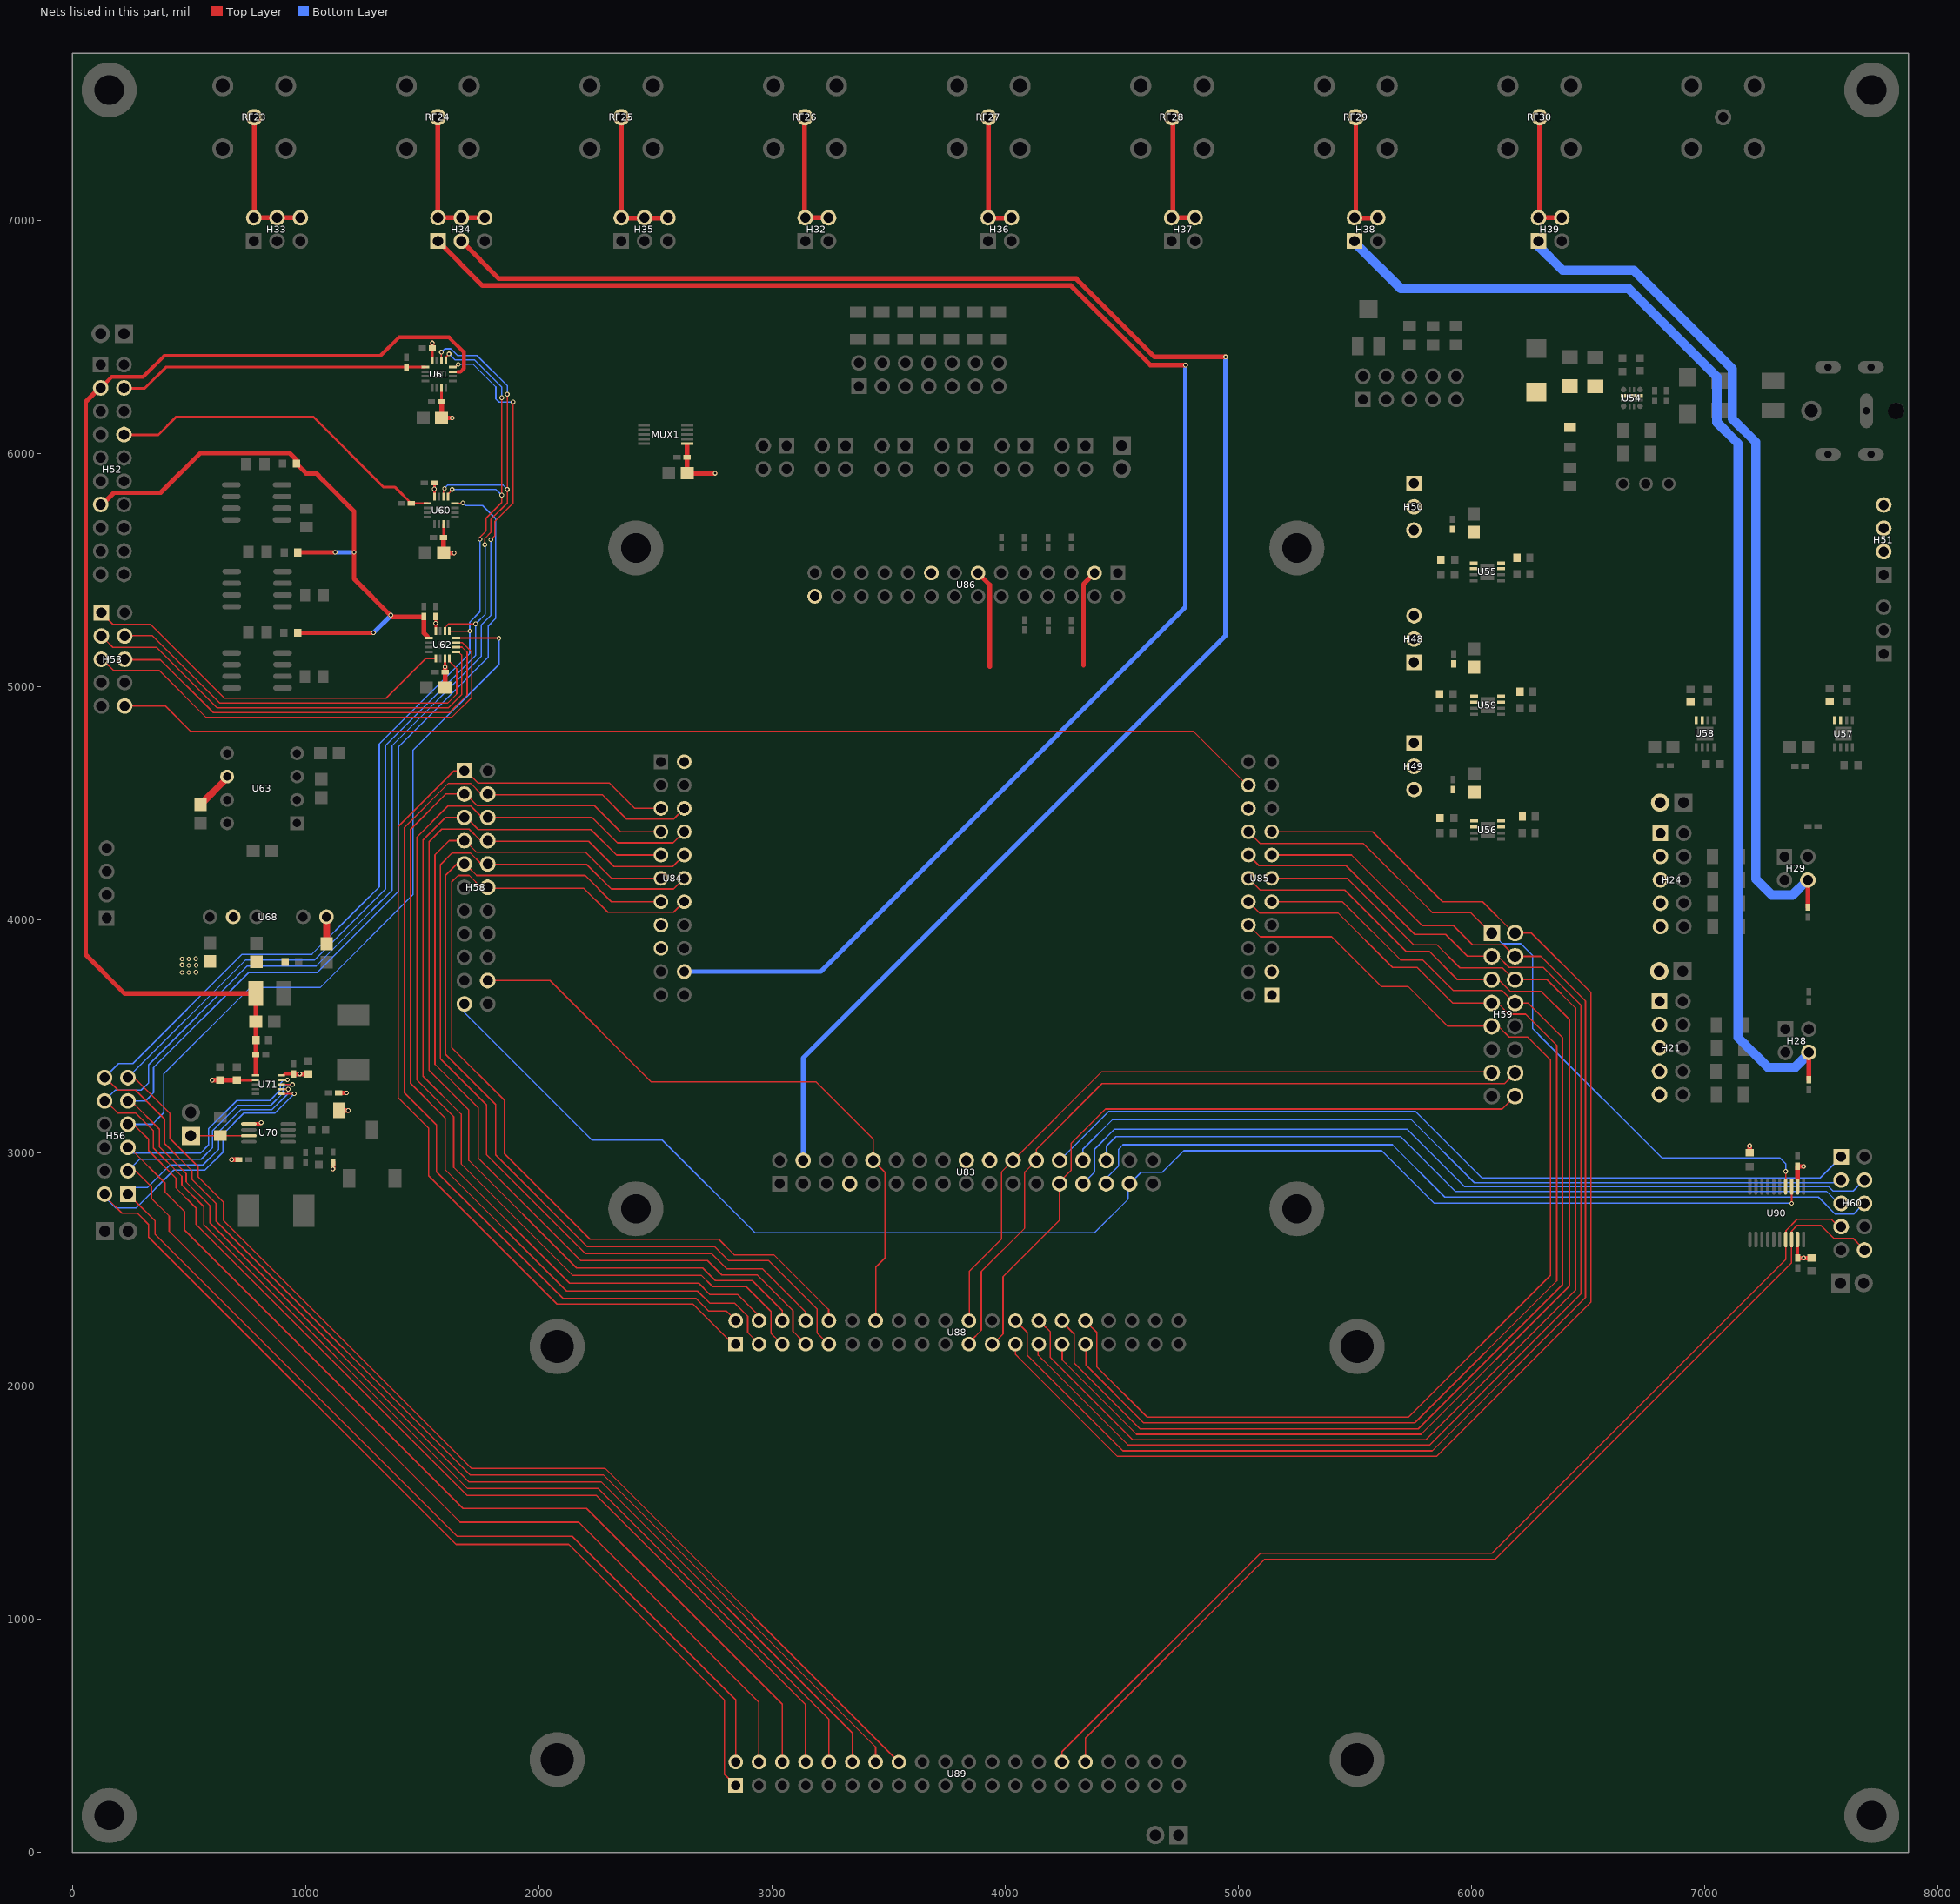
[diagram p0: the nets of this part, all layers, seen from the top]
# Altium PCB MISC62793.pcbdoc (part 3 of 6)
Units mil, origin at the board's own origin, x right, y up, seen from the top; angles counter-clockwise.
Board outline 7874.02 x 7716.54 mil, 4 copper layers (Top Layer, GND, VCC, Bottom Layer); 201 components, 197 nets, 941 pads, 1215 vias.

## Part data
C126: library part CC0603KRX7R9BB103
C129 C132 C135 C138 C141 C183 C193: library part CL10A105KO8NNNC
C130 C133 C136 C140 C143: library part CC0603JRX7R7BB103
C131 C134 C137 C139 C142 C144 C145 C146 C147 C148 C149 C150 C151 C152: library part C1210X475J5RAC7800
C157 C158 C159: library part CC0402KRX5R7BB154
C160 C161 C162 C163 C185 C186 C187: library part CL21A475KBQNNNE
C182 C215 C217: library part CC0402KRX7R7BB104
C184: library part EMK325ABJ107MM-P
C188: library part CC0402FRNPO9BN680
C189: library part GJM1555C1H240FB01D
C190 C191 C192 C196 C198 C199 C202 C203 C204 C205 C206 C207 C208 C219 C221 C223 C225 C226 C227: library part CL05B104KO5NNNC
C194 C195: library part CC0603KRX7R9BB102
C197 C218 C220 C224 C228: library part CL21A106KOQNNNE
C200 C201: library part CL31A226KAHNNNE
C216: library part CL05A105KO5NNNC
D4: library part VS-10BQ015HM3/5BT
D5: library part SMAJ12CA_C908818
H1 H2 H3 H4 H22 H23 H47 H57: library part X6511WV-02H-C60D30
H21 H24 H30: library part X6521WV-2x05H-C60D30
H27 H48 H49 H50: library part X6511WV-03H-C60D30
H28 H29 H32 H36 H37 H38 H39 H40 H41 H42 H43 H44 H45: library part PZ254-2-02-Z-8.5_C2894963
H33 H34 H35: library part PZ254-2-03-Z-8.5_C2894964
H46: library part PZ254-2-07-Z-8.5
H51 H54: library part X6511WV-04H-C60D30
H52: library part X6521WV-2x10H-C60D30
H53 H60: library part PZ254-2-05-Z-8.5_C2894966
H56: library part PZ254-2-06-Z-8.5
H58: library part PZ254-2-11-Z-8.5
H59: library part PZ254-2-08-Z-8.5
L5: library part ACM7060-301-2PL-TL01
L6 L7: library part FXL0630-100-M
MUX1: library part TMUX1104DGSR
R91 R93 R96 R97 R98: library part 0603WAF1002T5E
R92: library part 0603WAF5232T5E
R94: library part FRC0603F3092TS
R95: library part 0402WGF1252TCE
R99 R103: library part 1206W4F100KT5E
R100 R104: library part 1206W4F100JT5E
R101 R105: library part 1206W4F1000T5E
R102 R106: library part 1206W4F100LT5E
R108 R109 R110 R128 R137: library part RT0603BRD0710KL
R111 R112 R113 R114 R115 R116: library part 0805W8F2002T5E
R117: library part ARG05FTC4001N
R118: library part ARG05BTC5001N
R119: library part "ST-32EA 200K ohm (204)"
R120 R121 R122 R123 R124 R125 R126 R133: library part 1206W4F1004T5E
R127: library part 0603WAF0000T5E
R129 R130 R135: library part RT0805BRD071KL
R131: library part RT0603BRD07100KL
R132: library part RT0603BRD07100RL
R134: library part RT0603BRD07681RL
RF23 RF24 RF25 RF26 RF27 RF28 RF29 RF30 RF31: library part DOSIN-801-0057
SW2: library part K3-1204D
SW3: library part ST-5ETW503
U53: library part "HX DC007B-2.5"
U54: library part TPS259472ARPWR
U55 U56 U57 U58 U59: library part TPS7A8001DRBR
U60 U61 U62: library part DAC80508ZRTER
U63: library part MAX680CPA+
U64 U65 U66: library part OPA192IDR
U67: library part 0805W8F8001T5E
U68: library part A0505S-1WR3_C131042
U70: library part AD8512ARMZ-REEL
U71: library part ADS8881IDRCT
U82: library part RT1206BRD07357KL
U83: library part PM254-2-17-Z-8.5
U84 U85: library part PM254-2-11-Z-8.5
U86: library part PM254-2-14-Z-8.5
U88 U89: library part PM254-2-20-Z-8.5
U90: library part NXS0108PW-Q100J

## Free pads (board coordinates)
  round 236.22 hole 125.98: 0(157.48,157.48) 0(157.48,7559.06) 0(7716.54,157.48) 0(7716.54,7559.06) 2(2416.33,2760.14) 2(2416.33,5594.79) 2(5250.98,2760.14) 2(5250.98,5594.79)
  round 236.22 hole 141.73: 0(2079.05,397.63) 0(2079.05,2169.28) 0(5509.76,397.63) 0(5509.76,2169.28)

## Via types
v1: diameter 20, hole 12, Top Layer to Bottom Layer, 1215 vias

## Nets (pads, with @x,y where several pads share a name; then routed paths per layer and width w, separated by ;. In a path a pad name is that pad's centre, name@x,y a point inside that pad or via, vN(x,y) a via of type N, cw(c..) or ccw(c..) an arc to the next point about the centre after c; other vN are vias at no path point)
0V: C186.2 C187.2 C188.2 C190.2 C191.1 R127.1 R132.1 U68.5 U70.5 | length 190.2
  Top Layer w14: U70.5@756.5,3124.44 804.44,3124.44 v1(810,3130)
  Top Layer w20: v1(683,2971) C190.2@713.54,2971 ; v1(1116.99,2931.01) C188.2@1116.99,2960.59 ; C191.1@1141.46,3257 v1(1175,3257) ; R132.1@1142.22,3182 v1(1183,3182)
  other v1: 470,3774 499,3774 530,3775 499,3804 531,3805 470,3806 470,3832 499,3832 529,3833
1P8V: C137.2 C146.2 C215.2 H49.1 H49.2 H49.3 R95.2 R137.1 U56.1 U56.2 U83.26 U84.2 U84.17 U85.1 U85.18 U90.2 | length 117.5
  Top Layer w20: R137.1@7193,3000.66 v1(7193,3030) ; U90.2@7398.71,2889 7398.71,2902 ; 7398.71,2912 7398.71,2902 ; C215.2@7399.34,2942 C215.2@7400,2942 ; v1(7424,2942) C215.2@7400,2942 ; 7398.71,2902 7398.71,2940.71 C215.2@7400,2942
3P3V: C134.2 C145.2 C183.2 C192.1 C193.1 C194.1 C216.2 C217.2 C223.2 C226.2 C227.2 H48.1 H48.2 H48.3 R94.1 U59.1 U59.2 U60.16 U61.16 U62.16 U71.2 U71.10 U86.17 U86.28 U90.19 | length 630.2
  Top Layer w12: C193.1@633.99,3312.49 C194.1@705.99,3312.49 768.49,3312.49 ; U71.10@907,3334 911.44,3338.44 C192.1@951.44,3338.44 ; U61.16@1543.17,6415 C226.2@1543.17,6443.83 ; v1(1552,5847) v1@1552.6,5847 ; U60.16@1552.6,5815.31 v1@1552.6,5847 ; C223.2@1552.6,5865.4 v1@1552.6,5847 ; v1(1558,5272) v1@1558.22,5272 ; 1558.22,5256 v1@1558.22,5272 ; C227.2@1558.22,5292.22 v1@1558.22,5272
  Top Layer w13: C217.2@7398.71,2552.29 U90.19@7398.71,2628.68
  Top Layer w20: v1(598.51,3312.49) C194.1@705.99,3312.49 ; C192.1@951.44,3338.44 v1@975,3338.44 ; v1(975,3339) v1@975,3338.44 ; C183.2@1011,3338.44 v1@975,3338.44 ; C226.2@1543.46,6453 v1(1543.46,6473.46) ; C217.2@7405.44,2548.56 v1@7424,2548.56 ; v1(7424,2549) v1@7424,2548.56 ; C216.2@7458,2548.56 v1@7424,2548.56
  Bottom Layer w20: H48.1@5748,5095 5748,5091 H48.1@5756.5,5082.5
5V: C129.2 C132.2 C135.2 C138.2 C141.2 C200.2 C201.2 D4.1 H51.2 H51.3 H51.4 LED2.2 U54.6 U55.7 U55.8 U56.7 U56.8 U57.7 U57.8 U58.7 U58.8 U59.7 U59.8
ADC_1_OUT0: H60.1 U83.22 | length 3563.7
  Bottom Layer w6: U83.22@4233.65,2967.63 4443.03,3177 5760,3177 6045,2892 7495,2892 H60.1@7564,2961
ADC_1_OUT1: H60.4 U83.14 | length 3611.5
  Bottom Layer w6: U83.14@4333.65,2867.63 4384,2917.97 4384,3016 4470,3102 5723,3102 5970,2855 7512,2855 7532,2855 7550,2837 7637,2837 H60.4@7668,2868
ADC_1_OUT2: H60.3 U83.21 | length 3475.4
  Bottom Layer w6: U83.21@4333.65,2967.63 4333.65,3015.65 4461,3143 5741,3143 6012,2872 7491,2872 ; 7522,2872 7491,2872 ; H60.3@7565,2872 7491,2872
ADC_1_OUT3: H60.6 U83.15 | length 3498.6
  Bottom Layer w6: U83.15@4433.65,2867.63 4433.65,2891.65 4486,2944 4486,3015 4506,3035 5661,3035 5886,2810 7473,2810 7488,2810 7560,2738 7639,2738 H60.6@7671,2770
ADC_1_OUT4: H60.5 U83.20 | length 3327.1
  Bottom Layer w6: U83.20@4433.65,2967.63 4433.65,3028.65 4475,3070 5696,3070 5932,2834 7524,2834 H60.5@7567,2791
ADC_CNV: H56.2 U71.6 U89.1 | length 5084
  Top Layer w6: H56.2@150,2804 213,2741 279,2741 327,2693 327,2639 1645,1321 2128,1321 2796,653 2796,335.4 U89.1@2844.4,287 ; U71.6@895.31,3253.65 v1(951.65,3253.65)
  Bottom Layer w6: H56.2@144,2806 186,2764 273,2764 435,2926 568,2926 645,3003 645,3080 735,3170 868,3170 v1(951.65,3253.65)
ADC_DIN: H56.5 U71.9 U89.6 | length 4984.9
  Top Layer w6: H56.5@258,3015 258,3009 397,2870 397,2832 481,2748 481,2669 1132,2018 ; U71.9@895.31,3312.7 921.7,3312.7 v1(922,3313) ; 1129,2021 1132,2018 ; U89.6@3044.4,387 3044.4,635.6 2205,1475 1675,1475 1132,2018
  Bottom Layer w6: H56.5@252,3008 261,2999 549,2999 584,3034 584,3104 705,3225 847,3225 891,3269 891,3297 907,3313 v1(922,3313)
ADC_EN: H59.14 U83.23 U88.21 | length 3099
  Top Layer w6: U88.21@3852,2193 3898,2239 3898,2491 4084,2677 4084,2917.97 U83.23@4133.65,2967.63 4133.65,3014.65 4416,3297 6142,3297 H59.14@6167,3322
ADC_OUT: H56.1 U71.7 U89.2 | length 4681.7
  Top Layer w6: H56.1@267,2796 355,2708 355,2650 1650,1355 2143,1355 2844.4,653.6 U89.2@2844.4,387 ; U71.7@895.31,3273.33 v1(925.33,3273.33)
  Bottom Layer w6: H56.1@266,2851 322,2851 419,2948 560,2948 627,3015 627,3089 724,3186 856,3186 923,3253 923,3271 v1@924,3272
ADC_OUT0: H59.9 U85.8 U88.32 | length 4955.2
  Top Layer w6: U88.32@4356,2267 4393,2230 4393,2082 4609,1866 5022,1866 ; 5014,1866 5022,1866 ; U85.8@5043.5,3977.46 5093.96,3927 5400,3927 5613,3714 5728,3714 5899,3543 H59.9@6087,3543 6116,3543 6162,3497 6241,3497 6339,3399 6339,2475 5730,1866 5022,1866
ADC_OUT1: H59.8 U85.9 U88.30 | length 5193
  Top Layer w6: U88.30@4251,2268 4296,2223 4296,2099 4579,1816 5772,1816 6391,2435 6391,3494 6242,3643 H59.8@6187,3643 ; U85.9@5143.5,4077.46 5446.54,4077.46 5696,3828 5790,3828 5922,3696 6131,3696 H59.8@6178,3649
ADC_OUT2: H59.7 U85.10 U88.31 | length 5040.8
  Top Layer w6: U88.31@4346,2168 4346,2090 4594,1842 5757,1842 6366,2451 6366,3461 6232,3595 6160,3595 6112,3643 H59.7@6087,3643 5919,3643 5767,3795 5662,3795 5429,4028 5092.96,4028 U85.10@5043.5,4077.46
ADC_OUT3: H59.6 U85.11 U88.28 | length 5557
  Top Layer w6: U88.28@4160,2266 4193,2233 4193,2190 4193,2123 4547,1769 5804,1769 6446,2411 6446,3621 6324,3743 H59.6@6187,3743 ; U85.11@5143.5,4177.46 5466.54,4177.46 5751,3893 5851,3893 5951,3793 6133,3793 H59.6@6180,3746
ADC_OUT4: H59.5 U85.12 U88.29 | length 5400.7
  Top Layer w6: U88.29@4245,2171 4245,2112 4260,2097 4564,1793 5784,1793 6421,2430 6421,3571 6299,3693 6166,3693 6116,3743 H59.5@6087,3743 5940,3743 5819,3864 5719,3864 5456,4127 5093.96,4127 U85.12@5043.5,4177.46
ADC_OUT5: H59.4 U85.13 U88.26 | length 5860
  Top Layer w6: U88.26@4056,2269 4095,2230 4095,2190 4095,2132 4505,1722 5832,1722 6489,2379 6489,3652 6298,3843 H59.4@6187,3843 ; U85.13@5143.5,4277.46 5485.54,4277.46 5789,3974 5923,3974 6005,3892 6137,3892 H59.4@6182,3847
ADC_OUT6: H59.3 U85.14 U88.27 | length 5727.3
  Top Layer w6: U88.27@4139,2165 U88.27@4139,2169 ; U88.27@4142,2165 4142,2132 4158.5,2115.5 4162.5,2111.5 4528,1746 5820,1746 6469,2395 6469,3634 6308,3795 6162,3795 6114,3843 H59.3@6087,3843 ; U85.14@5043.5,4277.46 5088.96,4232 5462,4232 5757,3937 5889,3937 5982,3844 6020,3844 ; 6033,3844 6020,3844 ; H59.3@6078,3844 6020,3844
ADC_OUT7: H59.2 U85.15 U88.25 | length 5939.5
  Top Layer w6: U88.25@4044,2162 4044,2136 4066,2114 ; 4047,2133 4066,2114 ; U85.15@5143.5,4377.46 5575.54,4377.46 5876,4077 6048,4077 H59.2@6172,3953 ; H59.2@6187,3943 6257,3943 6512,3688 6512,2360 5850,1698 4482,1698 4066,2114
ADC_REF: C184.2 C195.2 C196.1 C197.2 H52.3 U61.11 U71.1 | length 5378.8
  Top Layer w11: H52.3@127,6286 127,6285 H52.3@128,6284 ; U61.11@1631.75,6350.28 1653,6350.28
  Top Layer w16: H52.3@121,6281 168.46,6328.46 303.46,6328.46 394,6419 1321,6419 1400,6498 1615,6498 1679,6434 1679,6365 1664.45,6350.45 1653,6350.45
  Top Layer w20: H52.3@104,6268 57,6221 57,3850 223.95,3683.05 C184.2@786.25,3683.05 786.25,3339.25
ADC_RST: H59.16 U83.13 U88.23 | length 2950.6
  Top Layer w6: U88.23@3958,2190 3991,2223 3991,2224 3991,2469 4233.65,2711.65 U83.13@4233.65,2867.63 ; U83.13@4244,2886 4283,2925 4283,3041 4430,3188 6132,3188 H59.16@6187,3243
ADC_SCLK: H56.3 U71.8 U89.4 | length 4928.9
  Top Layer w6: H56.3@252,2921 273,2921 340,2854 340,2804 415,2729 415,2664 1098,1981 ; U71.8@895.31,3293.02 v1(943.98,3293.02) ; 1094,1985 1098,1981 ; U89.4@2944.4,387 2944.4,642.6 2171,1416 1663,1416 1098,1981
  Bottom Layer w6: H56.3@238,2923 288,2973 552,2973 601,3022 601,3095 710,3204 851,3204 904,3257 904,3280 917.02,3293.02 v1(943.98,3293.02)
ADC_SL: H47.1 R130.2 U70.7 | length 234.2
  Top Layer w6: H47.1@522.26,3073.26 U70.7@756.5,3073.26
ADC_TEST_EN: H59.1 U85.16 U90.4 | length 3203
  Top Layer w6: U85.16@5043.5,4377.46 5093.96,4327 5536,4327 5832,4031 5996,4031 H59.1@6074,3953 ; H59.1@6087,3943 6089,3943 H59.1@6120,3912 ; U90.4@7347.53,2854.74 v1(7347.53,2920.53)
  Bottom Layer w6: H59.1@6087,3943 6133,3897 6212,3897 6262,3847 6262,3533 6312.5,3482.5 6817,2978 7323,2978 7348,2953 v1@7348,2923
ADC_TEST_EN_3V3: H60.7 U89.30 U90.17 | length 4390.6
  Top Layer w6: U89.30@4244.4,387 4244.4,432.4 5094,1282 6087,1282 7347.53,2542.53 U90.17@7347.53,2628.68 U90.17@7347.53,2656 ; U90.17@7349,2656 7349,2667 7397,2715 7543,2715 H60.7@7564,2694
AVDD: H23.2 H24.1 H24.3 H24.5 H24.7 H24.9 U86.3 U86.13 | length 837.2
  Top Layer w20: U86.13@3883.65,5487.31 3934,5436.96 3934,5086 ; 4336,5092 4336,5439.65 U86.3@4383.65,5487.31
BL_TEST: H53.10 U85.20 | length 4957.6
  Top Layer w6: H53.10@236,4922 242,4916 297,4916 ; 273,4916 297,4916 ; U85.20@5030,4585 4806,4809 506,4809 399,4916 297,4916
BNC1: H33.2 H33.4 H33.6 RF23.1 | length 628.3
  Top Layer w20: H33.2@774,7019 782,7011 H33.4@877.64,7011 H33.6@977.64,7011 ; H33.2@779.64,7020.64 RF23.1@779.64,7441.99
BNC2: H34.2 H34.4 H34.6 RF24.1 | length 615.2
  Top Layer w20: RF24.1@1567.04,7441.99 1567.04,7019.04 1575.09,7011 H34.4@1668,7011 H34.6@1756,7011
BNC3: H35.2 H35.4 H35.6 RF25.1 | length 646.9
  Top Layer w20: RF25.1@2354.45,7441.99 2354.45,7013.55 2359,7009 H35.6@2571,7009
BNC4: H32.2 H32.4 RF26.1 | length 527
  Top Layer w20: RF26.1@3139,7442 3139,7024 3152,7011 H32.4@3242.61,7011
BNC5: H36.2 H36.4 RF27.1 | length 519.8
  Top Layer w20: RF27.1@3929.25,7441.99 3929.25,7016.75 3936,7010 H36.4@4021,7010
BNC6: H37.2 H37.4 RF28.1 | length 525
  Top Layer w20: RF28.1@4705,7435 4719,7421 4719,7087 4719,7011 H37.4@4814.21,7011
BNC7: H38.2 H38.4 RF29.1 | length 534.7
  Top Layer w20: RF29.1@5504.05,7441.99 5504.05,7008.95 5599.95,7008.95 H38.4@5604,7013
BNC8: H39.2 H39.4 RF30.1 | length 519
  Top Layer w20: RF30.1@6291.45,7441.99 6291.45,7014.55 6294,7012 H39.4@6382,7012
BNC_AVDD: C152.2 H29.4 H39.1 | length 3667.2
  Top Layer w20: C152.2@7443,4053.46 H29.4@7443,4153
  Bottom Layer w40: H39.1@6287.61,6911 6287.61,6889.39 6391,6786 6696,6786 7119,6363 7119,6149 7219,6049 7219,4175 7288,4106 7377,4106 H29.4@7434,4163
BNC_DVDD: C150.2 H28.4 H38.1 | length 5128
  Top Layer w20: C150.2@7447,3314.46 H28.4@7447,3413
  Bottom Layer w40: H38.1@5506,6898 5696,6708 6673,6708 7052,6329 7052,6134 7143,6043 7143,4970 7143,3495 7273,3365 7386,3365 H28.4@7442,3421
CAL: H59.13 U83.24 U88.22 | length 2966.8
  Top Layer w6: U88.22@3846,2291 3846,2341 ; 3846,2323 3846,2341 ; H59.13@6071,3347 4413.03,3347 U83.24@4033.65,2967.63 3984,2917.97 3984,2629 3846,2491 3846,2341
CD: H34.3 U83.33 | length 7691.5
  Top Layer w20: H34.3@1668,6911 1829,6750 4305,6750 4641,6414 v1(4945,6414)
  Bottom Layer w20: U83.33@3133.65,2967.63 3133.65,3406.65 4945,5218 4945,6295 ; 4945,6308 4945,6295 ; v1@4945,6413 4945,6295
CLK: H58.20 U83.30 U88.14 | length 2752.5
  Top Layer w6: H58.20@1781,3739 2048,3739 2482,3305 3189,3305 3433.65,3060.35 U83.30@3433.65,2967.63 3485,2916.28 3485,2549 3446,2510 3446,2341 ; U88.14@3446,2292 3446,2341 ; 3446,2328 3446,2341
COL_ADDR0: H58.10 U84.12 U88.8 | length 4175.9
  Top Layer w6: H58.10@1781,4239 1754,4239 1706,4287 1629,4287 1578,4236 1578,3404 1776,3206 1776,2992 2200,2568 2741,2568 2807,2502 2960,2502 3111,2351 ; H58.10@1784,4253 1799,4238 2205,4238 2311,4132 2578.35,4132 U84.12@2623.81,4177.46 ; 3123,2339 3111,2351 ; U88.8@3144,2285 3144,2318 3111,2351
COL_ADDR1: H58.7 U84.11 U88.7 | length 4191.8
  Top Layer w6: H58.7@1681,4339 1615,4339 1555,4279 1555,3380 1741,3194 1741,2977 2180,2538 2724,2538 2785,2477 2937,2477 3090,2324 3090,2235 U88.7@3132,2193 ; H58.7@1693,4330 1734,4289 2201,4289 2312.54,4177.46 U84.11@2523.81,4177.46
COL_ADDR2: H58.8 U84.10 U88.6 | length 4292.6
  Top Layer w6: H58.8@1781,4339 1751,4339 1701,4389 1584,4389 1530,4335 1530,3354 1700,3184 1700,2968 2162,2506 2703,2506 2757,2452 2916,2452 3044.4,2323.6 U88.6@3044.4,2279.91 ; H58.8@1788,4346 1798,4336 2214,4336 2322,4228 2574.35,4228 U84.10@2623.81,4277.46 ; U88.6@3043,2279 U88.6@3043,2279.91
COL_ADDR3: H58.5 U84.9 U88.5 | length 4294.6
  Top Layer w6: H58.5@1681,4439 1601,4439 1504,4342 1504,3329 1667,3166 1667,2953 2146,2474 2698,2474 2746,2426 2890,2426 2996,2320 2996,2226 U88.5@3034,2188 ; H58.5@1703,4425 1741,4387 2224,4387 2333.54,4277.46 U84.9@2523.81,4277.46
COL_ADDR4: H58.6 U84.8 U88.4 | length 4350.2
  Top Layer w6: H58.6@1781,4439 1757,4439 1709,4487 1610,4487 1477,4354 1477,3313 1635,3155 1635,2938 2132,2441 2686,2441 2734,2393 2853,2393 2918.5,2327.5 ; H58.6@1784,4444 1789,4439 2228,4439 2337,4330 2576.35,4330 U84.8@2623.81,4377.46 ; 2923,2323 2918.5,2327.5 ; U88.4@2947,2299 2918.5,2327.5
COL_ADDR5: H58.3 U84.7 U88.3 | length 4383.7
  Top Layer w6: H58.3@1681,4539 1601,4539 1449,4387 1449,3299 1598,3150 1598,2929 2119,2408 2681,2408 2734,2355 2840,2355 2896,2299 2896,2229 U88.3@2937,2188 ; H58.3@1702,4523 1736,4489 2239,4489 2350.54,4377.46 U84.7@2523.81,4377.46
COL_ADDR6: H58.4 U84.6 U88.2 | length 4426.5
  Top Layer w6: H58.4@1781,4539 1754,4539 1708,4585 1613,4585 1423,4395 1423,3258 1561,3120 1561,2919 2104,2376 2674,2376 2729,2321 2806,2321 U88.2@2838,2289 ; H58.4@1789,4543 1796,4536 2273,4536 2377,4432 2578.35,4432 U84.6@2623.81,4477.46
COL_ADDR7: H58.1 U84.5 U88.1 | length 4520.6
  Top Layer w6: H58.1@1681,4639 1636,4639 1397,4400 1397,3237 1528,3106 1528,2902 2078,2352 2661,2352 2713.5,2299.5 ; H58.1@1708,4618 1739,4587 2302,4587 2411.54,4477.46 U84.5@2523.81,4477.46 ; 2795,2218 2713.5,2299.5 ; U88.1@2830,2192 2821,2192 2713.5,2299.5
COL_ADDR_EN: H58.9 U84.13 U88.9 | length 4089.6
  Top Layer w6: H58.9@1681,4239 1649,4239 1601,4191 1601,3422 1815,3208 1815,2991 2208,2598 2754,2598 2814,2538 2986,2538 3193,2331 3193,2228 U88.9@3231,2190 ; H58.9@1694,4230 1734,4190 2199,4190 2311.54,4077.46 U84.13@2523.81,4077.46
COL_CTRL: H58.12 U84.14 U88.10 | length 4067.4
  Top Layer w6: H58.12@1781,4139 1753,4139 1702,4190 1654,4190 1627,4163 1627,3451 1852,3226 1852,2997 2220,2629 2772,2629 2838,2563 3008,2563 3217,2354 ; H58.12@1797,4138 1800,4135 2193,4135 2296,4032 2578.35,4032 U84.14@2623.81,4077.46 ; 3237,2334 3217,2354 ; U88.10@3243,2292 3243,2328 3217,2354
DAC3_OUT3: H53.1 U62.5 | length 1634
  Top Layer w6: H53.1@140,5301 174,5267 335,5267 652,4950 1345,4950 1514.95,5119.95 U62.5@1558.22,5119.95
DAC3_OUT4: H53.4 U62.8 | length 1715
  Top Layer w6: H53.4@234,5219 342,5219 632,4929 1609,4929 1648,4968 1648,5077 1617.27,5107.73 U62.8@1617.27,5119.95
DAC3_OUT5: H53.3 U62.9 | length 1870.9
  Top Layer w6: H53.3@141,5201 174,5168 361,5168 620,4909 1613,4909 1669,4965 1669,5136 1655.53,5149.47 U62.9@1646.8,5149.47
DAC3_OUT6: H53.6 U62.10 | length 1822.9
  Top Layer w6: H53.6@234,5115 377,5115 604,4888 1617,4888 1693,4964 1693,5147 1670.84,5169.16 U62.10@1646.8,5169.16
DAC3_OUT7: H53.5 U62.11 | length 1986.7
  Top Layer w6: H53.5@138,5107 176,5069 372,5069 574,4867 1626,4867 1712,4953 1712,5149 1672.16,5188.84 U62.11@1646.8,5188.84
DAC_CS1: H56.9 U60.12 U89.12 | length 8010
  Top Layer w6: H56.9@258,3216 373,3101 373,3026 488,2911 488,2875 589,2774 589,2700 1701,1588 2269,1588 3344.4,512.6 U89.12@3344.4,387 ; U60.12@1641.18,5785.78 1672.78,5785.78 1674,5787 v1(1674,5788)
  Bottom Layer w6: H56.9@238,3223 313,3223 348,3258 348,3366 755,3773 1049,3773 1399,4123 1399,4742 1783,5126 1783,5260 1815,5292 1815,5720 1759,5776 1686,5776 v1(1674,5788)
DAC_CS2: H56.10 U61.12 U89.10 | length 8810.4
  Top Layer w6: H56.10@156,3210 195,3171 271,3171 347,3095 347,3021 469,2899 469,2863 563,2769 563,2692 1695,1560 2255,1560 3244.4,570.6 U89.10@3244.4,387 ; U61.12@1631.75,6369.97 1641.97,6369.97 1654,6382 v1(1655,6382) ; v1(1794,5630) 1812,5648 1812,5709 1890,5787 1890,6047 ; 1890,6059 1890,6047 ; v1(1890,6221) v1@1890,6218 ; v1@1891,6219 v1@1890,6218 ; 1890,6047 v1@1890,6218
  Bottom Layer w6: H56.10@138,3223 184,3269 295,3269 326,3300 326,3378 750,3802 1046,3802 1279,4035 1282,4038 1370,4126 1370,4746 1754,5130 1754,5264 1794,5304 v1(1794,5630) ; v1(1655,6382) 1719,6382 1816,6285 1816,6234 1830,6220 1887,6220 v1@1889,6222
DAC_CS3: H56.7 U62.12 U89.8 | length 7426.2
  Top Layer w6: H56.7@260,3124 289,3095 ; 285,3099 289,3095 ; 1174.5,2049.5 1179,2045 ; U62.12@1646.8,5208.53 v1@1829,5208.53 ; U89.8@3144.4,387 3144.4,633.6 2247,1531 1693,1531 1179,2045 ; 289,3095 326,3058 326,3010 445,2891 445,2849 530,2764 530,2694 1179,2045
  Bottom Layer w6: H56.7@238,3123 343,3123 392,3172 392,3339 762,3709 1062,3709 1460,4107 1460,4726 1830,5096 v1@1830,5202
  other v1: 1829,5207
DAC_REF1: C157.2 H52.8 U60.1 | length 1477.7
  Top Layer w11: H52.8@223,6080 368,6080 444,6156 1034,6156 1335,5855 1384.01,5855 C157.2@1453.78,5785.23 ; C157.2@1461.22,5785.78 U60.1@1523.07,5785.78
DAC_REF2: C158.2 H52.4 U61.1 | length 1315.9
  Top Layer w11: H52.4@235,6280 311,6280 400.97,6369.97 U61.1@1513.64,6369.97
DAC_REF3: C159.2 H52.13 R108.1 R109.1 R110.1 U62.1 | length 2698.9
  Top Layer w20: H52.13@133,5787 177.54,5831.54 378.54,5831.54 548.5,6001.5 931.5,6001.5 961.05,5971.95 R108.1@961.05,5957.07 R108.1@967.56,5950.56 ; R109.1@961,5574 R109.1@963,5576 ; R110.1@966.78,5231.07 v1(1290.93,5231.07) ; R108.1@967,5950 1002,5915 1045,5915 1074,5886 1081,5879 1208,5752 v1(1208,5576) 1208,5462 1371,5299 C159.2@1506,5299 ; R109.1@967.05,5576 v1(1127,5576) ; C159.2@1506.74,5300.55 1506.74,5230.26 U62.1@1523,5214
  Bottom Layer w20: v1(1127,5576) v1(1208,5576) ; v1(1290.93,5231.07) v1(1365.86,5306)
DAC_SCLK: H56.12 U60.13 U61.13 U62.13 U89.14 | length 9187.9
  Top Layer w6: H56.12@156,3309 196,3269 270,3269 395,3144 395,3040 512,2923 512,2887 616,2783 616,2708 1705,1619 2277,1619 3444.4,451.6 U89.14@3444.4,387 ; U61.13@1602.22,6399.5 1602.22,6414.22 v1(1615,6427) ; U60.13@1611.65,5815.31 1611.65,5826.65 v1@1628,5843 ; U62.13@1617.27,5238.06 v1(1703.94,5238.06) ; v1@1748,5641 1774,5667 1774,5722 1841,5789 v1@1841,5815 ; v1(1841,5821) v1(1841,6239)
  Bottom Layer w6: H56.12@138,3323 198,3383 259,3383 728,3852 1027,3852 1228,4053 1231,4056 1316,4141 1316,4754 1704,5142 v1(1703.94,5238.06) ; v1(1615,6427) 1641,6401 1725,6401 1841,6285 v1(1841,6239) ; v1(1628,5846) 1816,5846 v1(1841,5821) ; v1(1703.94,5238.06) 1703.94,5276.94 1748,5321 v1(1748,5632)
DAC_SDI: H56.11 U60.14 U61.14 U62.14 U89.16 | length 9305.3
  Top Layer w6: H56.11@255,3317 270.46,3317 418,3169.46 418,3062 539,2941 539,2897 647,2789 647,2711 1247,2111 ; 1244.5,2113.5 1247,2111 ; U61.14@1582.54,6399.5 v1(1582.54,6434.54) ; U60.14@1591.97,5815.31 v1@1591.97,5844.97 ; U62.14@1597.59,5238.06 1597.59,5253.35 1613.24,5269 v1(1729,5269) ; v1(1769,5608) 1769,5636 1794,5661 1794,5717 1865,5788 v1(1865,5846) v1@1865,6248 ; U89.16@3544.4,387 2284.4,1647 1711,1647 1247,2111
  Bottom Layer w6: H56.11@238,3323 743,3828 1039,3828 1343,4132 1343,4748 1730,5135 1730,5234 ; v1(1582.54,6434.54) 1597,6449 1623,6449 1652,6420 1735,6420 1866,6289 v1@1866,6255 ; v1@1597,5852 1610,5865 1846,5865 v1(1865,5846) ; v1(1729,5269) 1771,5311 1771,5606 v1(1769,5608) ; 1730,5239 1730,5234 ; v1@1730,5265 1730,5234
  other v1: 1596,5849 1865,6254
DAC_VDD: C131.2 C144.2 C162.1 C182.2 C185.1 C218.2 C219.2 C220.2 C221.2 C224.2 C225.2 C228.2 H50.1 H50.2 H50.3 MUX1.6 R92.2 U55.1 U55.2 U60.7 U61.7 U62.7 U63.6 U68.1 | length 959.6
  Top Layer w11: C221.2@1582.54,6227.46 U61.7@1582.54,6281.39 ; C219.2@1591.97,5641.03 U60.7@1591.97,5697.2 ; v1@1597.59,5083.8 v1@1597.59,5084 ; U62.7@1597.59,5119.95 v1@1597.59,5084 ; v1(1598,5084) v1@1597.59,5084
  Top Layer w20: C220.2@1583.06,6152.44 v1(1628.56,6152.44) ; C220.2@1583.15,6147.85 C221.2@1583.15,6221.44 ; C219.2@1591.69,5634.69 C218.2@1591.69,5573.23 v1(1636.77,5573.23) ; C224.2@1598.2,4999.8 C225.2@1598.2,5062.01 v1@1598.2,5083.8 ; 2636.37,6035.63 C228.2@2636.37,5915 v1(2756,5915)
  Top Layer w30: C162.1@549,4493.37 658.63,4603 U63.6@663,4603 ; C185.1@1090,3896.37 U68.1@1090,4000
DRIVER_TEST: H58.21 U83.16 U90.3 | length 6448.8
  Top Layer w6: v1(7373.12,2783.12) U90.3@7373.12,2854.74
  Bottom Layer w6: H58.21@1681,3639 1681,3602 2228,3055 2530,3055 2928,2657 4383,2657 4528,2802 U83.16@4528,2854 ; U83.16@4533.65,2867.63 4583.03,2917 4674,2917 4766,3009 5615,3009 5839,2785 v1@7372,2785
DRIVER_TEST_3V3: H60.10 U89.32 U90.18 | length 4430.9
  Top Layer w6: U89.32@4344.4,387 4344.4,489.4 5112,1257 6101,1257 7372,2528 U90.18@7372,2603 ; U90.18@7373.12,2628.68 7373.12,2665.12 7397,2689 7498,2689 7554,2633 7637,2633 H60.10@7671,2599
DVDD: H21.1 H21.3 H21.5 H21.7 H21.9 H22.2 U83.4 U83.25 U84.15 U85.3
EGD: H34.1 U84.20 | length 7261.2
  Top Layer w20: H34.1@1568,6911 1759,6720 4282,6720 4623,6379 v1(4774,6379)
  Bottom Layer w20: U84.20@2623.81,3777.46 3209.46,3777.46 4773,5341 v1@4773,6379